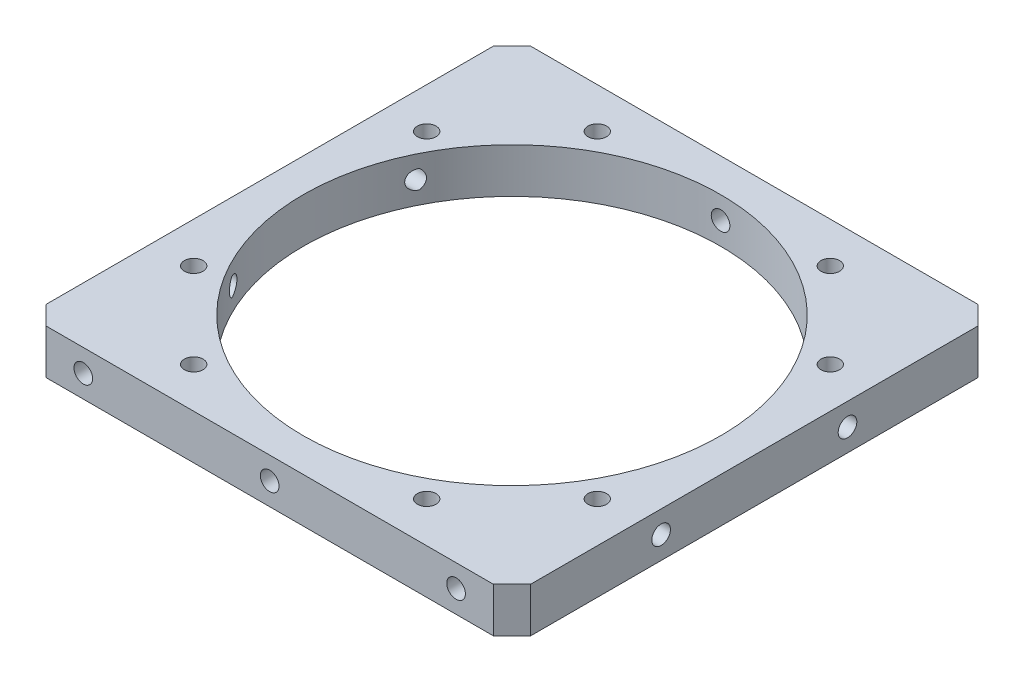
SolidWorks part; units mm, degrees
material "6061Al"
ref_plane "前视基准面" through (0, 0, 0) normal (0, 0, 1) x (1, 0, 0)
ref_plane "上视基准面" through (0, 0, 0) normal (0, 1, 0) x (1, 0, 0)
ref_plane "右视基准面" through (0, 0, 0) normal (1, 0, 0) x (0, 0, -1)
sketch "草图1" plane through (0, 0, 0) normal (0, 1, 0) x (1, 0, 0)
  line L1 (-65, -65) -> (65, -65)
  line L2 (-65, -65) -> (-65, 65)
  line L3 (-65, 65) -> (65, 65)
  line L4 (65, -65) -> (65, 65)
  line L5 (-65, -65) -> (65, 65) construction
  line L6 (-65, 65) -> (65, -65) construction
  point P0 (0, 0)
  dimension "D1" = 130
extrude "凸台-拉伸1" add sketch "草图1" along normal blind 12
sketch "草图2" plane through (0, 12, 0) normal (0, 1, 0) x (1, 0, 0)
  circle A0 centre (0, 0) radius 56
  dimension "D1" = 112
extrude "切除-拉伸1" cut sketch "草图2" against normal through all
hole_wizard "M6 螺纹孔1" positions "草图3" profile "草图4" tap size "M6" standard "GB"
sketch "草图3" plane through (0, 12, 0) normal (0, 1, 0) x (1, 0, 0)
  line L0 (0, 0) -> (31.25, 54.1266) construction
  point P0 (31.25, 54.1266)
  point P7 (54.1266, 31.25)
  point P9 (54.1266, -31.25)
  point P10 (31.25, -54.1266)
  point P12 (-31.25, -54.1266)
  point P13 (-54.1266, -31.25)
  point P15 (-54.1266, 31.25)
  point P16 (-31.25, 54.1266)
  point P24 (0, 62.5) [skipped]
  point P25 (62.5, 0) [skipped]
  point P26 (0, -62.5) [skipped]
  point P27 (-62.5, 0) [skipped]
  dimension "D1" = 12
sketch "草图4" plane through (31.25, 12, -54.1266) normal (1, 0, 0) x (0, 0, 1)
  line L0 (0, 0) -> (0, 12)
  line L1 (0, 12) -> (2.5, 12)
  line L2 (2.5, 12) -> (2.5, 0)
  line L5 (2.5, 0) -> (0, 0)
  line L11 (0, -6.35) -> (0, 107.95) construction
  dimension "通孔螺纹孔钻头直径" = 5
  dimension "通孔螺纹孔钻头深度" = 12
cosmetic thread "孔螺蚊线1" parameters "D2"=6
cosmetic thread "孔螺蚊线2" parameters "D2"=6
cosmetic thread "孔螺蚊线3" parameters "D2"=6
cosmetic thread "孔螺蚊线4" parameters "D2"=6
cosmetic thread "孔螺蚊线5" parameters "D2"=6
cosmetic thread "孔螺蚊线6" parameters "D2"=6
cosmetic thread "孔螺蚊线7" parameters "D2"=6
cosmetic thread "孔螺蚊线8" parameters "D2"=6
hole_wizard "M6 螺纹孔2" positions "草图5" profile "草图6" tap size "M6" standard "GB"
sketch "草图5" plane through (65, 0, 0) normal (1, 0, 0) x (0, 0, -1)
  line L0 (0, 12) -> (0, 0) construction
  line L1 (-65, 12) -> (65, 12) construction
  line L3 (0, 6) -> (65, 6) construction
  line L4 (65, 12) -> (65, 0) construction
  point P0 (-25, 6)
  point P2 (25, 6)
  dimension "D1" = 50
sketch "草图6" plane through (65, 6, 25) normal (0, 1, 0) x (0, 0, -1)
  line L0 (0, 0) -> (0, 16.5022)
  line L1 (0, 16.5022) -> (2.5, 15)
  line L2 (2.5, 15) -> (2.5, 0)
  line L5 (2.5, 0) -> (0, 0)
  line L10 (0, 16.5022) -> (-2.5, 15) construction
  line L11 (0, -6.35) -> (0, 107.95) construction
  dimension "螺纹孔钻头直径" = 5
  dimension "螺纹孔钻头深度" = 15
  dimension "导头角度" = 118
cosmetic thread "孔螺蚊线9" parameters "D1"=12, "D2"=6
cosmetic thread "孔螺蚊线10" parameters "D1"=12, "D2"=6
hole_wizard "M6 螺纹孔3" positions "草图7" profile "草图8" tap size "M6" standard "GB"
sketch "草图7" plane through (-65, 0, 0) normal (-1, 0, 0) x (0, 0, 1)
  point P0 (-25, 6)
  point P3 (25, 6)
sketch "草图8" plane through (-65, 6, -25) normal (0, 1, 0) x (0, 0, 1)
  line L0 (0, 0) -> (0, 16.5022)
  line L1 (0, 16.5022) -> (2.5, 15)
  line L2 (2.5, 15) -> (2.5, 0)
  line L5 (2.5, 0) -> (0, 0)
  line L10 (0, 16.5022) -> (-2.5, 15) construction
  line L11 (0, -6.35) -> (0, 107.95) construction
  dimension "螺纹孔钻头直径" = 5
  dimension "螺纹孔钻头深度" = 15
  dimension "导头角度" = 118
cosmetic thread "孔螺蚊线11" parameters "D1"=12, "D2"=6
cosmetic thread "孔螺蚊线12" parameters "D1"=12, "D2"=6
hole_wizard "M6 螺纹孔4" positions "草图9" profile "草图10" tap size "M6" standard "GB"
sketch "草图9" plane through (0, 0, -65) normal (0, 0, -1) x (-1, 0, 0)
  line L0 (0, 0) -> (0, 12) construction
  line L1 (-65, 12) -> (65, 12) construction
  line L3 (0, 6) -> (65, 6) construction
  line L4 (65, 12) -> (65, 0) construction
  point P0 (-50, 6)
  point P2 (50, 6)
  point P12 (0, 6)
  dimension "D1" = 100
sketch "草图10" plane through (50, 6, -65) normal (1, 0, 0) x (0, 1, 0)
  line L0 (0, 0) -> (0, 16.5022)
  line L1 (0, 16.5022) -> (2.5, 15)
  line L2 (2.5, 15) -> (2.5, 0)
  line L5 (2.5, 0) -> (0, 0)
  line L10 (0, 16.5022) -> (-2.5, 15) construction
  line L11 (0, -6.35) -> (0, 107.95) construction
  dimension "螺纹孔钻头直径" = 5
  dimension "螺纹孔钻头深度" = 15
  dimension "导头角度" = 118
cosmetic thread "孔螺蚊线13" parameters "D1"=12, "D2"=6
cosmetic thread "孔螺蚊线14" parameters "D1"=12, "D2"=6
cosmetic thread "孔螺蚊线17" parameters "D1"=12, "D2"=6
hole_wizard "M6 螺纹孔5" positions "草图11" profile "草图12" tap size "M6" standard "GB"
sketch "草图11" plane through (0, 0, 65) normal (0, 0, 1) x (1, 0, 0)
  point P0 (-50, 6)
  point P3 (50, 6)
  point P6 (0, 6)
sketch "草图12" plane through (-50, 6, 65) normal (1, 0, 0) x (0, -1, 0)
  line L0 (0, 0) -> (0, 16.5022)
  line L1 (0, 16.5022) -> (2.5, 15)
  line L2 (2.5, 15) -> (2.5, 0)
  line L5 (2.5, 0) -> (0, 0)
  line L10 (0, 16.5022) -> (-2.5, 15) construction
  line L11 (0, -6.35) -> (0, 107.95) construction
  dimension "螺纹孔钻头直径" = 5
  dimension "螺纹孔钻头深度" = 15
  dimension "导头角度" = 118
cosmetic thread "孔螺蚊线15" parameters "D1"=12, "D2"=6
cosmetic thread "孔螺蚊线16" parameters "D1"=12, "D2"=6
cosmetic thread "孔螺蚊线18" parameters "D1"=12, "D2"=6
chamfer "倒角1" distance 5 angle 45 4 edges at (-65, 6, 65) (65, 6, 65) (65, 6, -65) (-65, 6, -65)
